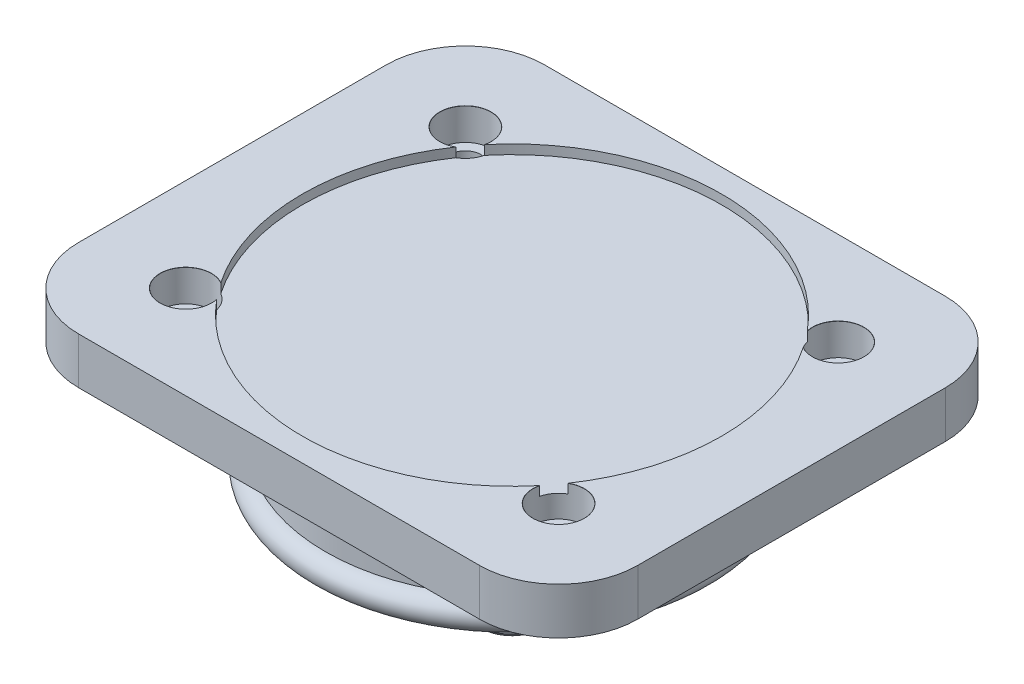
from build123d import *

# Parameters (mm, degrees)
BOSS_EXTRUDE1_DEPTH                          = 10
SKETCH2_R                                    = 40
BOSS_EXTRUDE2_DEPTH                          = 20
SKETCH3_R                                    = 3
CBORE_FOR_M6_HEXAGON_SOCKET_HEAD_CAP_2_COUNT = 2
CBORE_FOR_M6_HEXAGON_SOCKET_HEAD_CAP_2_PITCH = 80
CBORE_FOR_M6_HEXAGON_SOCKET_HEAD_CAP_3_COUNT = 2
CBORE_FOR_M6_HEXAGON_SOCKET_HEAD_CAP_3_PITCH = 100
CBORE_FOR_M6_HEXAGON_SOCKET_HEAD_CAP_4_COUNT = 2
CBORE_FOR_M6_HEXAGON_SOCKET_HEAD_CAP_4_PITCH = 60
SKETCH4_R                                    = 7.5
BOSS_EXTRUDE3_DEPTH                          = 25
CHAMFER1_SIZE                                = 1
SKETCH5_R                                    = 45
CUT_EXTRUDE1_DEPTH                           = 2


with BuildPart() as part:
    # Sketch1 → Boss-Extrude1 (new body)
    with BuildSketch(Plane(origin=(0, 0, 0), x_dir=(1, 0, 0), z_dir=(0, 1, 0))):
        with BuildLine():
            Line((-43, 50), (43, 50))
            ThreePointArc((43, 50), (55.02081528, 45.02081528), (60, 33))
            Line((60, 33), (60, -33))
            ThreePointArc((60, -33), (55.02081528, -45.02081528), (43, -50))
            Line((43, -50), (-43, -50))
            ThreePointArc((-43, -50), (-55.02081528, -45.02081528), (-60, -33))
            Line((-60, -33), (-60, 33))
            ThreePointArc((-60, 33), (-55.02081528, 45.02081528), (-43, 50))
        make_face()
    extrude(amount=BOSS_EXTRUDE1_DEPTH)

    # Sketch2 → Boss-Extrude2 (add)
    with BuildSketch(Plane.XZ):
        with Locations(Location((0, 0, 0), (0, 0, 270))):
            Circle(SKETCH2_R)
    extrude(amount=BOSS_EXTRUDE2_DEPTH)

    # Sketch3 → Revolve1 (revolve)
    with BuildSketch(Plane(origin=(0, 0, 0), x_dir=(0, 0, -1), z_dir=(1, 0, 0)), mode=Mode.PRIVATE) as revolve1_sk:
        with Locations((-40, -17)):
            Circle(SKETCH3_R)
    revolve(revolve1_sk.sketch.rotate(Axis((0, 22.515244343, 0), (0, -1, 0)), 180), axis=Axis((0, 22.515244343, 0), (0, -1, 0)))

    # Sketch9 → CBORE for M6 Hexagon socket head cap screws1 (revolve, cut)
    with BuildSketch(Plane(origin=(-40, 10, -30), x_dir=(0, 0, 1), z_dir=(1, 0, 0))):
        Polygon((0, 0), (0, 30), (3.3, 30), (3.3, 6.8), (5.5, 6.8), (5.5, 0.025), (5.525, 0), align=None)
    cbore_for_m6_hexagon_socket_head_cap_scr = revolve(axis=Axis((-40, 16.35, -30), (0, -1, 0)), mode=Mode.SUBTRACT)

    # CBORE for M6 Hexagon socket head cap 2: CBORE for M6 Hexagon socket head cap screws1 ×2
    with Locations(*[(i * CBORE_FOR_M6_HEXAGON_SOCKET_HEAD_CAP_2_PITCH, 0, 0) for i in range(1, CBORE_FOR_M6_HEXAGON_SOCKET_HEAD_CAP_2_COUNT)]):
        add(cbore_for_m6_hexagon_socket_head_cap_scr, mode=Mode.SUBTRACT)

    # CBORE for M6 Hexagon socket head cap 3: CBORE for M6 Hexagon socket head cap screws1 ×2
    with Locations(*[Vector(0.7999999999999999, 0, 0.6000000000000001) * (i * CBORE_FOR_M6_HEXAGON_SOCKET_HEAD_CAP_3_PITCH) for i in range(1, CBORE_FOR_M6_HEXAGON_SOCKET_HEAD_CAP_3_COUNT)]):
        add(cbore_for_m6_hexagon_socket_head_cap_scr, mode=Mode.SUBTRACT)

    # CBORE for M6 Hexagon socket head cap 4: CBORE for M6 Hexagon socket head cap screws1 ×2
    with Locations(*[(0, 0, i * CBORE_FOR_M6_HEXAGON_SOCKET_HEAD_CAP_4_PITCH) for i in range(1, CBORE_FOR_M6_HEXAGON_SOCKET_HEAD_CAP_4_COUNT)]):
        add(cbore_for_m6_hexagon_socket_head_cap_scr, mode=Mode.SUBTRACT)

    # Sketch4 → Boss-Extrude3 (add)
    with BuildSketch(Plane.XZ.offset(20)):
        with Locations(Location((0, 0, 0), (0, 0, 270))):
            Circle(SKETCH4_R)
    extrude(amount=BOSS_EXTRUDE3_DEPTH)

    # Chamfer1
    chamfer1_edges = [part.edges().sort_by_distance(p)[0] for p in [
        (0, -45, 7.5),
    ]]
    chamfer(chamfer1_edges, length=CHAMFER1_SIZE)

    # Sketch5 → Cut-Extrude1 (cut)
    with BuildSketch(Plane(origin=(0, 10, 0), x_dir=(1, 0, 0), z_dir=(0, 1, 0))):
        Circle(SKETCH5_R)
    extrude(amount=-CUT_EXTRUDE1_DEPTH, mode=Mode.SUBTRACT)


solid = part.part
